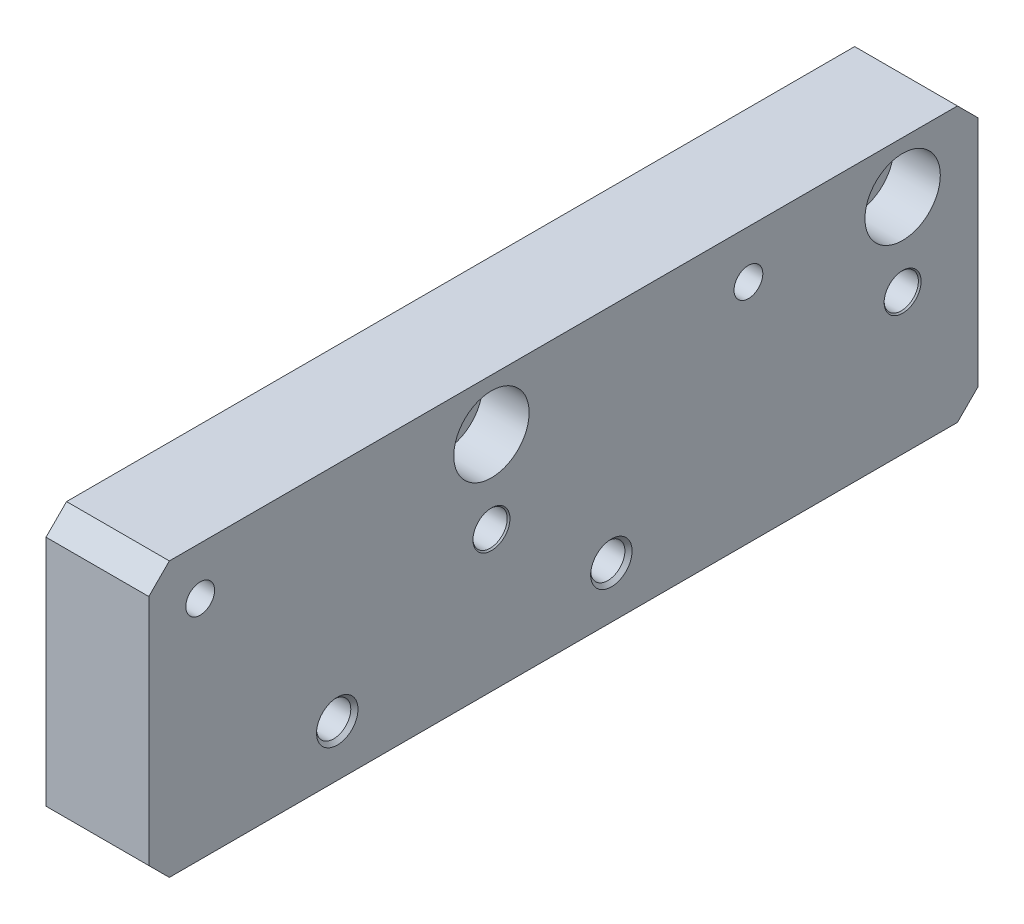
from build123d import *

# Parameters (mm, degrees)
SKETCH1_W                                            = 121
SKETCH1_H                                            = 40
BOSS_EXTRUDE1_DEPTH                                  = 15
M5_TAPPED_HOLE1_D                                    = 4.2
M5_TAPPED_HOLE1_DEPTH                                = 12.4
M5_TAPPED_HOLE1_TIP                                  = 1.2618073
M6_TAPPED_HOLE1_D                                    = 5
M6_TAPPED_HOLE1_DEPTH                                = 15
M6_TAPPED_HOLE1_CSINK_D                              = 6.05
M6_TAPPED_HOLE1_CSINK_ANGLE                          = 90
M6_TAPPED_HOLE1_TIP                                  = 1.502151548
CBORE_FOR_M6_HEXAGON_SOCKET_HEAD_CAP_SCR_D           = 6.6
CBORE_FOR_M6_HEXAGON_SOCKET_HEAD_CAP_SCR_CBORE_D     = 11
CBORE_FOR_M6_HEXAGON_SOCKET_HEAD_CAP_SCR_CBORE_DEPTH = 6.8
F_5_0MM_BLIND_HOLE_1_D                               = 5
F_5_0MM_BLIND_HOLE_1_CSINK_D                         = 5.4
F_5_0MM_BLIND_HOLE_1_CSINK_ANGLE                     = 90
CHAMFER1_SIZE                                        = 3


with BuildPart() as part:
    # Sketch1 → Boss-Extrude1 (new body)
    with BuildSketch(Plane(origin=(0, 0, 0), x_dir=(0, 0, -1), z_dir=(1, 0, 0))):
        Rectangle(SKETCH1_W, SKETCH1_H)
    extrude(amount=BOSS_EXTRUDE1_DEPTH)

    # M5 Tapped Hole1
    with Locations(Plane(origin=(15, 0, 0), x_dir=(0, 0, -1), z_dir=(1, 0, 0))):
        with Locations((-53, 13), (27, 13)):
            Hole(M5_TAPPED_HOLE1_D / 2, depth=M5_TAPPED_HOLE1_DEPTH)
            with Locations((0, 0, -(M5_TAPPED_HOLE1_DEPTH + M5_TAPPED_HOLE1_TIP / 2))):  # 118° drill point
                Cone(0, M5_TAPPED_HOLE1_D / 2, M5_TAPPED_HOLE1_TIP, mode=Mode.SUBTRACT)

    # M6 Tapped Hole1
    with Locations(Plane(origin=(15, 0, 0), x_dir=(0, 0, -1), z_dir=(1, 0, 0))):
        with Locations((-33, -12.5), (7, -12.5)):
            CounterSinkHole(M6_TAPPED_HOLE1_D / 2, M6_TAPPED_HOLE1_CSINK_D / 2, depth=M6_TAPPED_HOLE1_DEPTH, counter_sink_angle=M6_TAPPED_HOLE1_CSINK_ANGLE)
            with Locations((0, 0, -(M6_TAPPED_HOLE1_DEPTH + M6_TAPPED_HOLE1_TIP / 2))):  # 118° drill point
                Cone(0, M6_TAPPED_HOLE1_D / 2, M6_TAPPED_HOLE1_TIP, mode=Mode.SUBTRACT)

    # CBORE for M6 Hexagon socket head cap screws1 (through all)
    with Locations(Plane(origin=(15, 0, 0), x_dir=(0, 0, -1), z_dir=(1, 0, 0))):
        with Locations((-10.5, 12.5), (49.5, 12.5)):
            CounterBoreHole(CBORE_FOR_M6_HEXAGON_SOCKET_HEAD_CAP_SCR_D / 2, CBORE_FOR_M6_HEXAGON_SOCKET_HEAD_CAP_SCR_CBORE_D / 2, CBORE_FOR_M6_HEXAGON_SOCKET_HEAD_CAP_SCR_CBORE_DEPTH)

    # Ø5.0mm blind hole 1 (through all)
    with Locations(Plane(origin=(15, 0, 0), x_dir=(0, 0, -1), z_dir=(1, 0, 0))):
        with Locations((-10.5, 0.5), (49.5, 0.5)):
            CounterSinkHole(F_5_0MM_BLIND_HOLE_1_D / 2, F_5_0MM_BLIND_HOLE_1_CSINK_D / 2, counter_sink_angle=F_5_0MM_BLIND_HOLE_1_CSINK_ANGLE)

    # Chamfer1
    chamfer1_edges = [part.edges().sort_by_distance(p)[0] for p in [
        (7.5, -20, -60.5),
        (7.5, -20, 60.5),
        (7.5, 20, 60.5),
        (7.5, 20, -60.5),
    ]]
    chamfer(chamfer1_edges, length=CHAMFER1_SIZE)


solid = part.part
